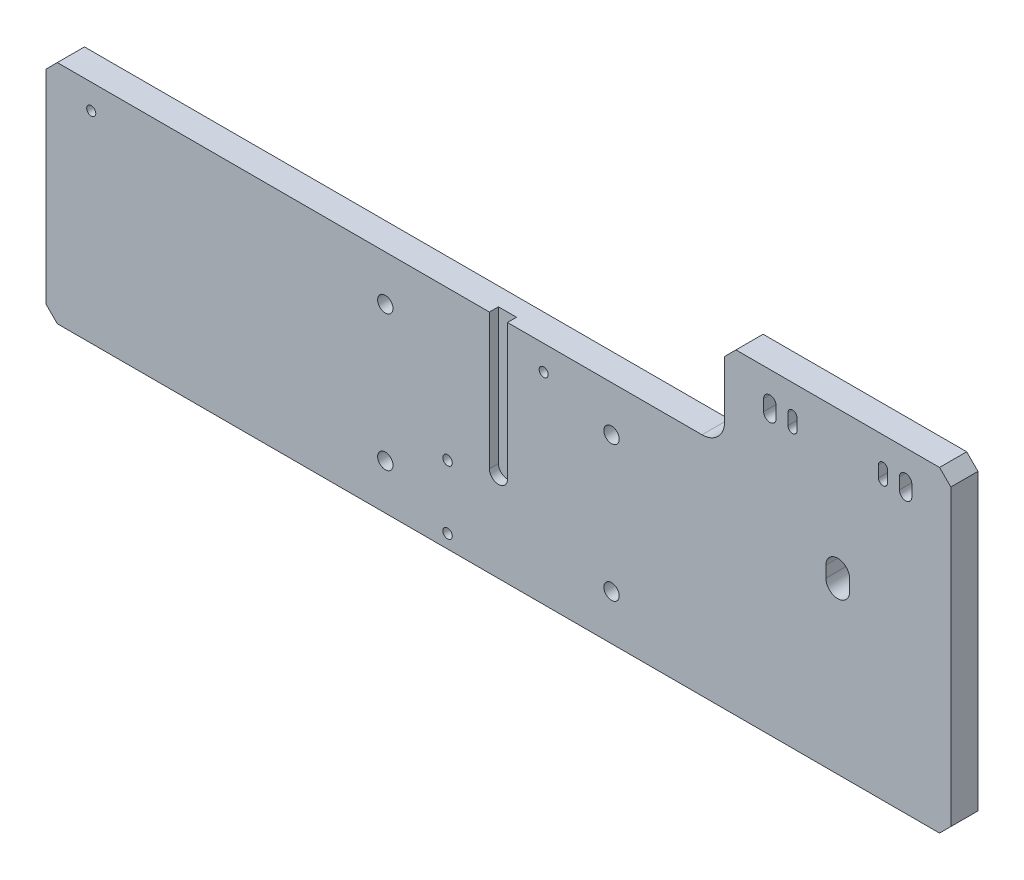
from build123d import *

# Parameters (mm, degrees)
SKETCH1_W                      = 400
SKETCH1_H                      = 100
BOSS_EXTRUDE1_DEPTH            = 12
SKETCH2_W                      = 100
SKETCH2_H                      = 12
BOSS_EXTRUDE2_DEPTH            = 40
CUT_EXTRUDE1_DEPTH             = 4
M8_TAPPED_HOLE2_D              = 6.8
M8_TAPPED_HOLE2_DEPTH          = 22
M8_TAPPED_HOLE2_TIP            = 2.042926105
M5_TAPPED_HOLE1_D              = 4.2
M5_TAPPED_HOLE1_DEPTH          = 12.4
M5_TAPPED_HOLE1_TIP            = 1.2618073
M4_TAPPED_HOLE1_D              = 3.3
M4_TAPPED_HOLE1_DEPTH          = 10.1
M4_TAPPED_HOLE1_TIP            = 0.991420021
SKETCH10_R                     = 2
CUT_EXTRUDE2_DEPTH             = 220.645168397
M8_TAPPED_HOLE1_D              = 6.8
M8_TAPPED_HOLE1_DEPTH          = 19.75
M8_TAPPED_HOLE1_TIP            = 2.042926105
F_5_5_5_5_DIAMETER_HOLE1_D     = 5.5
F_5_5_5_5_DIAMETER_HOLE1_DEPTH = 76
F_5_5_5_5_DIAMETER_HOLE1_TIP   = 1.652366702
CUT_EXTRUDE3_DEPTH             = 220.645168397
CHAMFER1_SIZE                  = 5
FILLET1_R                      = 10
CUT_EXTRUDE4_DEPTH             = 220.645168397


with BuildPart() as part:
    # Sketch1 → Boss-Extrude1 (new body)
    with BuildSketch(Plane.XY):
        Rectangle(SKETCH1_W, SKETCH1_H)
    extrude(amount=BOSS_EXTRUDE1_DEPTH)

    # Sketch2 → Boss-Extrude2 (add)
    with BuildSketch(Plane(origin=(0, 50, 0), x_dir=(1, 0, 0), z_dir=(0, 1, 0))):
        with Locations((150, -6)):
            Rectangle(SKETCH2_W, SKETCH2_H)
    extrude(amount=BOSS_EXTRUDE2_DEPTH)

    # Sketch3 → Cut-Extrude1 (cut)
    with BuildSketch(Plane.XY.offset(12)):
        with BuildLine():
            Line((4, 50), (4, -10))
            ThreePointArc((4, -10), (0, -14), (-4, -10))
            Line((-4, -10), (-4, 50))
            ThreePointArc((-4, 50), (0, 54), (4, 50))
        make_face()
    extrude(amount=-CUT_EXTRUDE1_DEPTH, mode=Mode.SUBTRACT)

    # M8 Tapped Hole2
    with Locations(Plane(origin=(0, -50, 0), x_dir=(-1, 0, 0), z_dir=(0, -1, 0))):
        with Locations((0, -6)):
            Hole(M8_TAPPED_HOLE2_D / 2, depth=M8_TAPPED_HOLE2_DEPTH)
            with Locations((0, 0, -(M8_TAPPED_HOLE2_DEPTH + M8_TAPPED_HOLE2_TIP / 2))):  # 118° drill point
                Cone(0, M8_TAPPED_HOLE2_D / 2, M8_TAPPED_HOLE2_TIP, mode=Mode.SUBTRACT)

    # M5 Tapped Hole1
    with Locations(Plane(origin=(0, 0, 0), x_dir=(-1, 0, 0), z_dir=(0, 0, -1))):
        with Locations((22.5, -16), (22.5, -44)):
            Hole(M5_TAPPED_HOLE1_D / 2, depth=M5_TAPPED_HOLE1_DEPTH)
            with Locations((0, 0, -(M5_TAPPED_HOLE1_DEPTH + M5_TAPPED_HOLE1_TIP / 2))):  # 118° drill point
                Cone(0, M5_TAPPED_HOLE1_D / 2, M5_TAPPED_HOLE1_TIP, mode=Mode.SUBTRACT)

    # M4 Tapped Hole1
    with Locations(Plane(origin=(0, 0, 0), x_dir=(-1, 0, 0), z_dir=(0, 0, -1))):
        with Locations((180, 25), (140, 25), (100, 25), (60, 25), (20, 25), (-20, 25)):
            Hole(M4_TAPPED_HOLE1_D / 2, depth=M4_TAPPED_HOLE1_DEPTH)
            with Locations((0, 0, -(M4_TAPPED_HOLE1_DEPTH + M4_TAPPED_HOLE1_TIP / 2))):  # 118° drill point
                Cone(0, M4_TAPPED_HOLE1_D / 2, M4_TAPPED_HOLE1_TIP, mode=Mode.SUBTRACT)

    # Sketch10 → Cut-Extrude2 (cut, through all)
    with BuildSketch(Plane(origin=(0, 0, 0), x_dir=(-1, 0, 0), z_dir=(0, 0, -1))):
        with Locations((180, 39)):
            Circle(SKETCH10_R)
        with Locations((-20, 39)):
            Circle(SKETCH10_R)
    extrude(amount=-CUT_EXTRUDE2_DEPTH, mode=Mode.SUBTRACT)

    # M8 Tapped Hole1
    with Locations(Plane(origin=(0, 0, 0), x_dir=(-1, 0, 0), z_dir=(0, 0, -1))):
        with Locations((50, -30), (50, 30), (-50, -30), (-50, 30)):
            Hole(M8_TAPPED_HOLE1_D / 2, depth=M8_TAPPED_HOLE1_DEPTH)
            with Locations((0, 0, -(M8_TAPPED_HOLE1_DEPTH + M8_TAPPED_HOLE1_TIP / 2))):  # 118° drill point
                Cone(0, M8_TAPPED_HOLE1_D / 2, M8_TAPPED_HOLE1_TIP, mode=Mode.SUBTRACT)

    # Ø5.5 (5.5) Diameter Hole1
    with Locations(Plane.XY.offset(12)):
        with Locations((120, 75), (180, 75), (150, 25)):
            Hole(F_5_5_5_5_DIAMETER_HOLE1_D / 2, depth=F_5_5_5_5_DIAMETER_HOLE1_DEPTH)
            with Locations((0, 0, -(F_5_5_5_5_DIAMETER_HOLE1_DEPTH + F_5_5_5_5_DIAMETER_HOLE1_TIP / 2))):  # 118° drill point
                Cone(0, F_5_5_5_5_DIAMETER_HOLE1_D / 2, F_5_5_5_5_DIAMETER_HOLE1_TIP, mode=Mode.SUBTRACT)

    # Sketch15 → Cut-Extrude3 (cut, through all)
    with BuildSketch(Plane.XY.offset(12)):
        with BuildLine():
            Line((122.75, 77.5), (122.75, 72.5))
            ThreePointArc((122.75, 72.5), (120, 69.75), (117.25, 72.5))
            Line((117.25, 72.5), (117.25, 77.5))
            ThreePointArc((117.25, 77.5), (120, 80.25), (122.75, 77.5))
        make_face()
        with BuildLine():
            Line((182.75, 77.5), (182.75, 72.5))
            ThreePointArc((182.75, 72.5), (180, 69.75), (177.25, 72.5))
            Line((177.25, 72.5), (177.25, 77.5))
            ThreePointArc((177.25, 77.5), (180, 80.25), (182.75, 77.5))
        make_face()
        with BuildLine():
            Line((155.25, 27.5), (155.25, 22.5))
            ThreePointArc((155.25, 22.5), (150, 17.25), (144.75, 22.5))
            Line((144.75, 22.5), (144.75, 27.5))
            ThreePointArc((144.75, 27.5), (150, 32.75), (155.25, 27.5))
        make_face()
    extrude(amount=-CUT_EXTRUDE3_DEPTH, mode=Mode.SUBTRACT)

    # Chamfer1
    chamfer1_edges = [part.edges().sort_by_distance(p)[0] for p in [
        (100, 90, 6),
        (200, 90, 6),
        (200, -50, 6),
        (-200, 50, 6),
        (-200, -50, 6),
    ]]
    chamfer(chamfer1_edges, length=CHAMFER1_SIZE)

    # Fillet1
    fillet1_edges = [part.edges().sort_by_distance(p)[0] for p in [
        (100, 50, 6),
    ]]
    fillet(fillet1_edges, radius=FILLET1_R)

    # Sketch16 → Cut-Extrude4 (cut, through all)
    with BuildSketch(Plane(origin=(0, 0, 0), x_dir=(-1, 0, 0), z_dir=(0, 0, -1))):
        with BuildLine():
            Line((-132, 72.5), (-132, 77.5))
            ThreePointArc((-132, 77.5), (-130, 79.5), (-128, 77.5))
            Line((-128, 77.5), (-128, 72.5))
            ThreePointArc((-128, 72.5), (-130, 70.5), (-132, 72.5))
        make_face()
        with BuildLine():
            Line((-172, 72.5), (-172, 77.5))
            ThreePointArc((-172, 77.5), (-170, 79.5), (-168, 77.5))
            Line((-168, 77.5), (-168, 72.5))
            ThreePointArc((-168, 72.5), (-170, 70.5), (-172, 72.5))
        make_face()
    extrude(amount=-CUT_EXTRUDE4_DEPTH, mode=Mode.SUBTRACT)


solid = part.part
